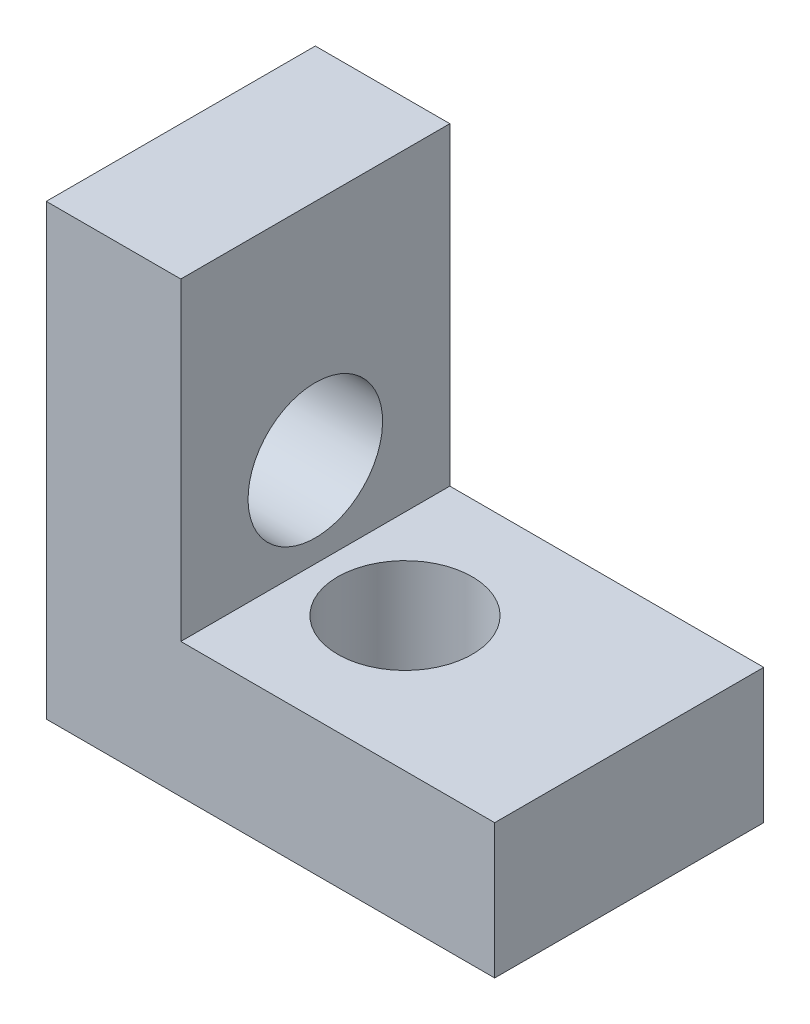
SolidWorks part; units mm, degrees
material "6061-O (SS)"
ref_plane "前视基准面" through (0, 0, 0) normal (0, 0, 1) x (1, 0, 0)
ref_plane "上视基准面" through (0, 0, 0) normal (0, 1, 0) x (1, 0, 0)
ref_plane "右视基准面" through (0, 0, 0) normal (1, 0, 0) x (0, 0, -1)
other "Configuration Table"
sketch "草图6" plane through (0, 0, 0) normal (0, 0, 1) x (1, 0, 0)
  line L0 (0, 0) -> (10, 0)
  line L1 (10, 0) -> (10, 3)
  line L2 (10, 3) -> (3, 3)
  line L3 (3, 3) -> (3, 10)
  line L4 (3, 10) -> (0, 10)
  line L5 (0, 10) -> (0, 0)
  dimension "D1" = 3
  dimension "D2" = 10
extrude "凸台-拉伸4" add sketch "草图6" along normal blind 6
sketch "草图7" plane through (3, 0, 0) normal (1, 0, 0) x (0, 0, -1)
  line L0 (-6, 3) -> (-6, 10) construction
  line L1 (-6, 10) -> (0, 10) construction
  circle A0 centre (-3, 5) radius 1.5
  dimension "D1" = 3
  dimension "D2" = 3
  dimension "D3" = 5
extrude "切除-拉伸3" cut sketch "草图7" against normal through all
sketch "草图8" plane through (0, 3, 0) normal (0, 1, 0) x (1, 0, 0)
  line L0 (10, 0) -> (3, 0) construction
  line L1 (10, -6) -> (10, 0) construction
  circle A0 centre (5, -3) radius 1.5
  dimension "D1" = 3
  dimension "D2" = 3
  dimension "D3" = 5
extrude "切除-拉伸4" cut sketch "草图8" against normal through all
